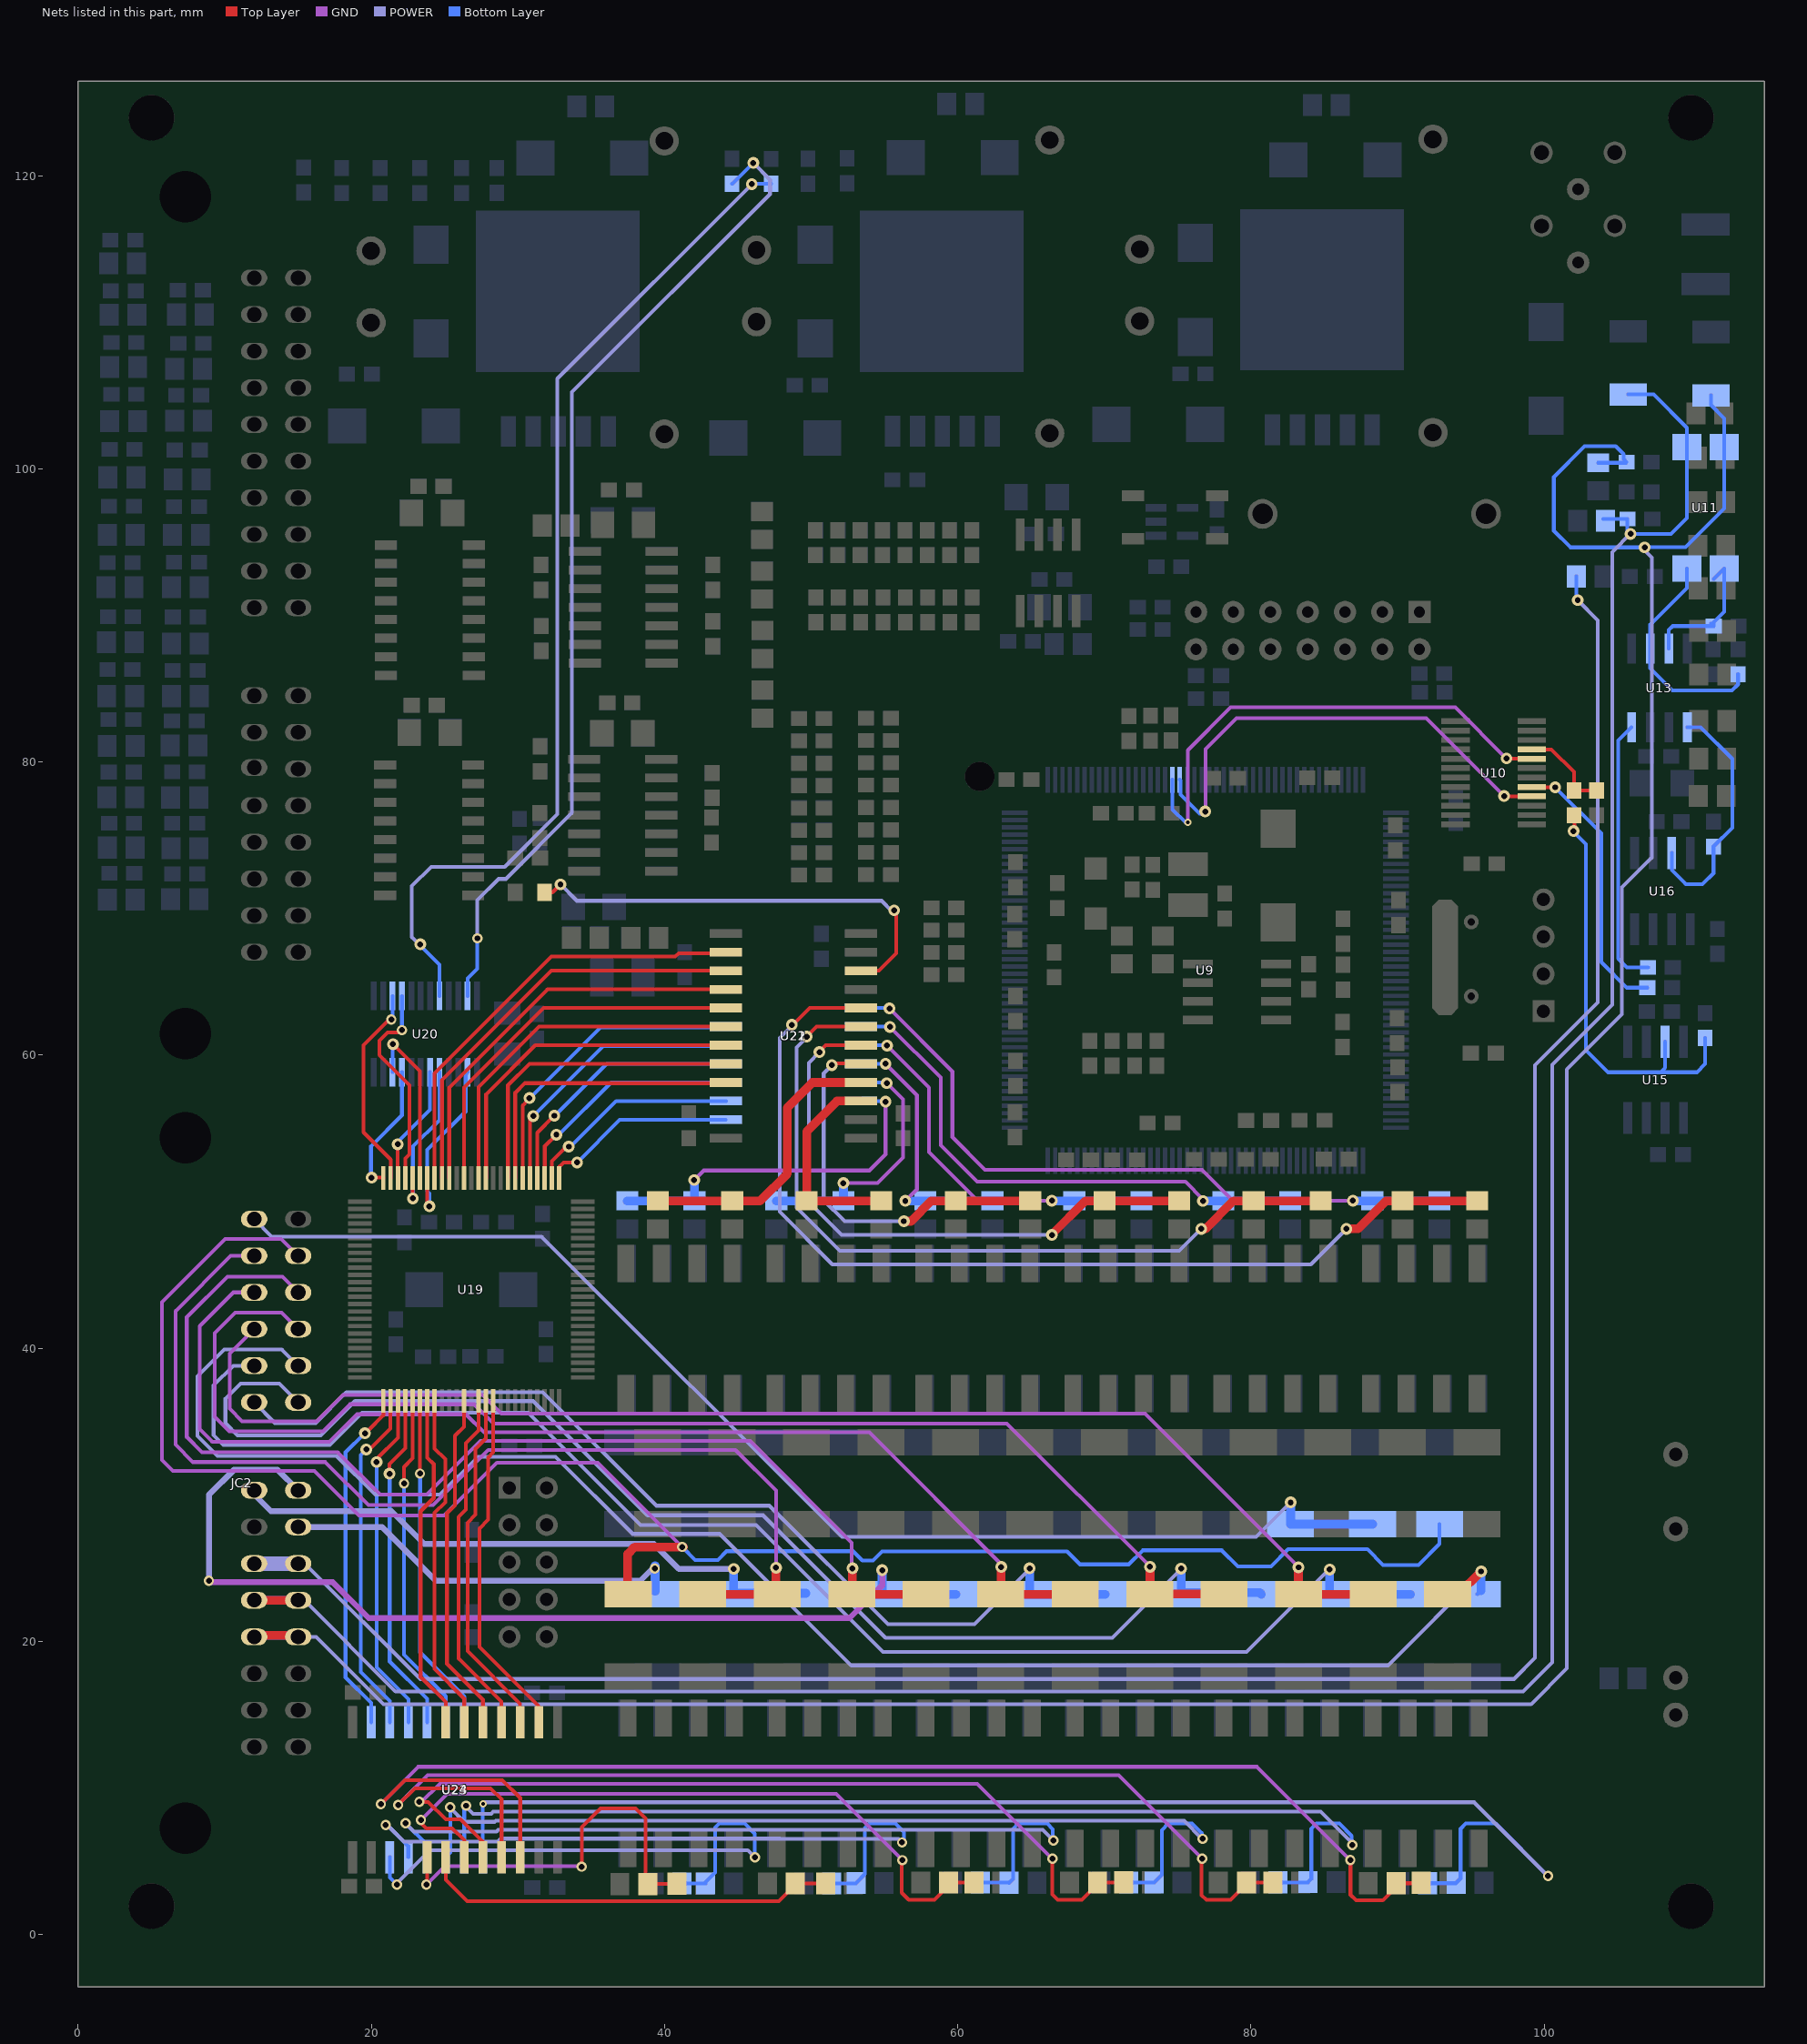
[diagram p0: the nets of this part, all layers, seen from the top]
# Altium PCB MISC86180.PCBDOC (part 5 of 9)
Units mm, origin at the board's own origin, x right, y up, seen from the top; angles counter-clockwise.
Board outline 115 x 130 mm, 4 copper layers (Top Layer, GND, POWER, Bottom Layer); 475 components, 355 nets, 1755 pads, 459 vias.

## Via types
v1: diameter 0.8, hole 0.4, Top Layer to Bottom Layer, 339 vias
v2: diameter 0.7, hole 0.4, Top Layer to Bottom Layer, 83 vias
v3: diameter 0.5, hole 0.254, Top Layer to Bottom Layer, 37 vias

## Nets (pads, with @x,y where several pads share a name; then routed paths per layer and width w, separated by ;. In a path a pad name is that pad's centre, name@x,y a point inside that pad or via, vN(x,y) a via of type N, cw(c..) or ccw(c..) an arc to the next point about the centre after c; other vN are vias at no path point) (continued)
BAT12: F22.1 F23.1 JC2.13 | length 87.7
  POWER w0.254: JC2.13@12.01,48.814 13.204,47.62 31.61,47.62 52.1,27.13 79.851,27.13 79.858,27.137 80.347,27.137 v1(82.7,29.49)
  Bottom Layer w0.254: v1@82.696,29.486 v1(82.7,29.49)
  Bottom Layer w0.6: v1(82.7,29.49) 82.7,28.01 88.28,28.01 F23.1@88.284,28.006
BAT13: F24.1 F25.1 JC2.4 | length 127.3
  Top Layer w0.254: v2@41.2,26.44 v2(41.2,26.45)
  Top Layer w0.6: F25.1@37.484,22.88 37.484,25.954 37.97,26.44 41.2,26.44 v2@41.3,26.44
  GND w0.254: JC2.4@15.01,46.314 13.854,47.47 10.03,47.47 5.71,43.15 5.71,32.39 6.46,31.64 16.11,31.64 19.15,28.6 24.97,28.6 28.57,32.2 35.44,32.2 41.19,26.45 v2(41.2,26.45) ; v2@41.215,26.465 41.22,26.46 v2@41.245,26.435
  Bottom Layer w0.254: v2@41.2,26.44 v2(41.2,26.45) 42.09,25.56 43.63,25.56 44.23,26.16 52.851,26.16 53.488,25.523 54.213,25.523 54.84,26.15 67.45,26.15 68.34,25.26 71.65,25.26 72.61,26.22 78,26.22 79.09,25.13 81.37,25.13 82.53,26.29 87.93,26.29 89,25.22 91.42,25.22 92.856,26.656 F24.1@92.856,28.006
BAT14: F26.1 F27.1 JC2.14 | length 73.7
  Top Layer w0.254: v1@47.6,24.78 v1(47.6,25.03)
  Top Layer w0.6: F26.1@42.604,23.22 F27.1@47.684,23.22 47.6,23.304 v1@47.6,24.78
  GND w0.254: JC2.14@12.01,46.314 10.414,46.314 6.64,42.54 6.64,33.43 7.83,32.24 16.86,32.24 19.8,29.3 24.21,29.3 26.895,31.985 27.98,33.07 44.83,33.07 47.6,30.3 v1(47.6,25.03) ; v1@47.56,25.01 v1@47.56,25.1
BAT15: F28.1 F29.1 JC2.5 | length 77.4
  Top Layer w0.6: v1(52.81,24.99) 52.81,23.266 52.856,23.22 F29.1@57.844,23.22
  GND w0.254: JC2.5@15.01,43.814 13.934,44.89 10.18,44.89 7.41,42.12 7.41,33.95 8.44,32.92 17.71,32.92 20.617,30.013 23.773,30.013 27.44,33.68 45.83,33.68 52.77,26.74 v1@52.77,24.91
BAT16: F30.1 F31.1 JC2.15 | length 78.8
  Top Layer w0.6: v1(62.96,25.08) 62.96,23.256 62.996,23.22 F31.1@68.004,23.22
  GND w0.254: JC2.15@12.01,43.814 10.594,43.814 8.3,41.52 8.3,34.48 9.15,33.63 17.15,33.63 19.02,35.5 26.46,35.5 27.69,34.27 53.97,34.27 62.92,25.32 v1@62.92,25.08
BAT17: F32.1 F33.1 JC2.6 | length 88.8
  Top Layer w0.6: v1(73.11,25.1) 73.11,23.246 78.138,23.246 F33.1@78.164,23.22
  GND w0.254: JC2.6@15.01,41.314 13.884,42.44 10.72,42.44 9.33,41.05 9.33,35.33 10.32,34.34 16.7,34.34 18.54,36.18 27.02,36.18 28.33,34.87 63.35,34.87 v1@73.07,25.15
BAT18: F34.1 F35.1 JC2.16 | length 91.9
  Top Layer w0.6: v1(83.23,25.06) 83.23,23.234 F34.1@83.244,23.22 F35.1@88.324,23.22
  GND w0.254: JC2.16@12.01,41.314 10.34,39.644 10.34,35.88 11.19,35.03 16.28,35.03 18.07,36.82 27.6,36.82 28.87,35.55 72.77,35.55 83.19,25.13 v1@83.19,25.09
BAT19: F36.1 F37.1 JC2.7 | length 115.6
  Top Layer w0.6: F36.1@93.404,23.22 94.13,23.22 v1(95.69,24.78)
  POWER w0.254: JC2.7@15.01,38.814 13.894,39.93 9.97,39.93 8.135,38.095 8.135,34.025 9.5,32.66 17.62,32.66 20.267,30.013 24.693,30.013 27.29,32.61 32.55,32.61 37.82,27.34 43.77,27.34 52.74,18.37 89.34,18.37 v1@95.735,24.765
  Bottom Layer w0.254: F37.1@95.436,23.22 F37.1@95.69,23.474
  Bottom Layer w0.6: F37.1@95.69,23.474 v1(95.69,24.78)
BAT20: F38.1 F39.1 JC2.17 | length 100.5
  POWER w0.254: JC2.17@12.01,38.814 10.584,38.814 9.24,37.47 9.24,34.08 9.92,33.4 17.18,33.4 19.38,35.6 30.71,35.6 38.36,27.95 46.25,27.95 54.91,19.29 79.7,19.29 v1@85.41,25
  Bottom Layer w0.254: F39.1@85.276,23.22 F39.1@85.444,23.22
  Bottom Layer w0.6: v1(85.36,24.91) 85.36,23.304 85.444,23.22 F38.1@90.864,23.22
BAT21: F40.1 F41.1 JC2.8 | length 89.9
  POWER w0.254: JC2.8@15.01,36.314 13.724,37.6 11.08,37.6 10.05,36.57 10.05,34.88 10.87,34.06 16.55,34.06 18.89,36.4 31.05,36.4 38.84,28.61 46.72,28.61 55.07,20.26 70.54,20.26 v1@75.225,24.945
  Bottom Layer w0.6: v1(75.23,24.97) 75.23,23.334 80.59,23.334 F40.1@80.704,23.22
BAT22: F42.1 F43.1 JC2.18 | length 69.4
  POWER w0.254: JC2.18@12.01,36.314 13.414,34.91 16.21,34.91 18.3,37 31.7,37 39.437,29.263 47.137,29.263 55.23,21.17 61.13,21.17 v1@64.96,25
  Bottom Layer w0.254: F43.1@64.9,23.276 F43.1@64.956,23.22
  Bottom Layer w0.6: F43.1@64.9,23.276 v1(64.9,24.99) ; F43.1@64.956,23.22 F42.1@70.036,23.22
BAT23: F44.1 F45.1 JC2.9 | length 69.2
  GND w0.4: v2(8.92,24.14) 9.01,24.05 17.36,24.05 19.82,21.59 52.61,21.59 54.84,23.82 v1(54.84,24.87)
  POWER w0.254: v1@54.74,24.82 v1@54.94,24.82
  POWER w0.4: v2(8.92,24.14) 8.92,30 10.65,31.73 13.594,31.73 JC2.9@15.01,30.314
  Bottom Layer w0.254: F45.1@54.796,23.22 F45.1@54.884,23.22
  Bottom Layer w0.6: v1(54.84,24.87) 54.84,23.264 54.884,23.22 F44.1@59.876,23.22
BAT24: F46.1 F47.1 JC2.19 | length 41.9
  POWER w0.4: JC2.19@12.01,30.314 12.01,30.03 13.154,28.885 21.375,28.885 23.605,26.655 39.265,26.655 40.97,24.95 v1(44.71,24.95)
  Bottom Layer w0.254: v1@44.636,24.876 v1(44.71,24.95) ; F46.1@49.642,23.22 F46.1@49.716,23.22
  Bottom Layer w0.6: v1(44.71,24.95) 44.71,23.294 F46.1@49.642,23.294
BAT25: F48.1 JC2.10 | length 27.9
  POWER w0.4: JC2.10@15.01,27.814 20.726,27.814 24.4,24.14 38.34,24.14 39.18,24.98 v2(39.33,24.98)
  Bottom Layer w0.254: v2@39.342,25.163 v2@39.349,25.17
  Bottom Layer w0.6: F48.1@39.35,23.426 v2@39.35,25.17
CAN1H: C60.2 DZ1.1 JC2.23 JC2.31 R17.2 U11.4 | length 209.4
  Top Layer w0.6: JC2.31@12.01,20.414 JC2.23@14.91,20.414
  POWER w0.254: JC2.23@15.01,20.314 16.236,20.314 20.83,15.72 99.1,15.72 101.54,18.16 101.54,52.89 ; 101.54,54.63 101.54,52.89 ; 105.29,69.915 105.29,71.39 105.3,71.4 105.3,71.44 107.34,73.48 107.34,93.942 106.85,94.432 v1(106.85,94.64) ; 105.3,69.861 105.3,62.78 101.54,59.02 101.54,52.89
  Bottom Layer w0.254: R17.2@103.672,100.409 105.557,100.409 C60.2@105.61,100.462 105.41,100.662 105.41,101 104.87,101.54 102.75,101.54 100.65,99.44 100.65,95.76 101.77,94.64 v1(106.85,94.64) ; v1@106.85,94.65 109.62,94.65 112.263,97.293 U11.4@112.263,101.485 112.263,103.447 111.36,104.35 DZ1.1@111.36,105.012
  Bottom Layer w0.6: JC2.31@12.01,20.414 JC2.23@14.91,20.414
CAN1HIN: C58.2 U11.1 U13.7 | length 9.9
  Bottom Layer w0.254: U13.7@108.49,87.727 108.49,89.01 108.752,89.272 C58.2@111.55,89.272 ; C58.2@111.382,89.44 C58.2@111.55,89.272 ; U11.1@111.55,92.472 U11.1@112.263,93.185 112.263,90.243 111.55,89.53 C58.2@111.55,89.272
CAN1L: C61.2 DZ2.1 JC2.22 JC2.30 R18.1 U11.3 | length 192.4
  Top Layer w0.6: JC2.30@12.01,22.814 JC2.22@15.01,22.814
  POWER w0.254: JC2.22@15.01,22.814 15.426,22.814 21.65,16.59 98.55,16.59 100.53,18.57 100.53,59.34 104.63,63.44 104.63,94.32 v1@105.95,95.64
  Bottom Layer w0.254: R18.1@104.019,96.582 C61.2@105.67,96.582 105.67,95.77 105.89,95.55 108.64,95.55 109.723,96.633 U11.3@109.723,101.485 109.723,102.799 107.45,105.072 DZ2.1@105.72,105.072
  Bottom Layer w0.6: JC2.30@12.01,22.814 JC2.22@15.01,22.814
  other v1: 105.89,95.56
CAN1LIN: C59.2 U11.2 U13.6 | length 15.3
  Bottom Layer w0.254: U11.2@109.723,93.185 109.723,91.863 107.23,89.37 107.23,87.737 U13.6@107.22,87.727 107.22,86.39 108.62,84.99 108.73,84.88 112.8,84.88 113.218,85.298 C59.2@113.218,85.99
CAN1RX: R22.2 U13.4 | length 18.5
  Bottom Layer w0.254: U13.4@105.95,82.377 105.03,81.457 105.03,66.59 105.63,65.99 107.062,65.99 R22.2@107.07,65.982
CAN1S: JC2.21 JC2.29 R19.2 | length 167.4
  POWER w0.254: JC2.21@15.01,25.314 15.476,25.314 23.35,17.44 97.93,17.44 99.37,18.88 99.37,59.32 103.65,63.6 103.65,89.67 v1(102.28,91.04)
  POWER w1: JC2.29@12.01,25.314 JC2.21@15.01,25.314
  Bottom Layer w0.254: R19.2@102.175,92.658 102.175,91.145 v1(102.28,91.04)
CAN1TX: R23.1 U13.1 U16.7 | length 17
  Bottom Layer w0.254: U16.7@108.693,73.791 108.693,72.617 109.65,71.66 110.79,71.66 111.542,72.412 R23.1@111.542,74.23 112.83,75.518 112.83,80.21 110.663,82.377 U13.1@109.76,82.377
CANAR: R13.1 R14.2 U10.9 | length 6.3
  Top Layer w0.254: U10.9@99.146,80.858 100.482,80.858 102.022,79.318 R13.1@102.022,78.06 R14.2@103.568,78.06
CANARR: R13.2 R21.1 U15.7 | length 29.6
  Top Layer w0.254: v1@101.82,75.11 v1@101.852,75.142 ; v1@102.07,75.16 R13.2@102.07,76.378
  Bottom Layer w0.254: v1@101.82,75.11 102.11,75.11 102.83,74.39 102.83,60.35 104.35,58.83 107.92,58.83 ; U15.7@108.231,60.913 108.231,59.141 107.92,58.83 ; R21.1@110.972,61.17 110.972,59.402 110.4,58.83 107.92,58.83
  other v1: 101.99,75.29
CANARX: U9.62 U10.8 | length 34.5
  Top Layer w0.254: v1(97.42,80.24) 97.442,80.218 U10.8@99.146,80.218
  GND w0.254: v3(75.68,75.87) 75.68,80.8 78.6,83.72 93.94,83.72 v1(97.42,80.24)
  Bottom Layer w0.254: U9.62@74.639,78.793 74.639,76.761 75.53,75.87 v3(75.68,75.87)
CANAT: R24.2 U10.5 | length 20.6
  Top Layer w0.254: U10.5@99.146,78.298 99.175,78.27 v1(100.74,78.27)
  Bottom Layer w0.254: v1(100.74,78.27) 103.88,75.13 103.88,66.34 105.618,64.602 ; 104.27,65.95 105.618,64.602 ; R24.2@107.02,64.602 105.618,64.602
CANATX: U9.63 U10.4 | length 33.4
  Top Layer w0.254: v1(97.26,77.67) 97.272,77.658 U10.4@99.146,77.658
  GND w0.254: v1(76.87,76.62) 77.026,76.464 76.9,76.59 76.9,80.88 79,82.98 91.95,82.98 v1(97.26,77.67)
  Bottom Layer w0.254: U9.63@75.139,78.793 75.184,78.748 75.184,77.778 76.499,76.463 76.838,76.463 76.87,76.496 v1(76.87,76.62)
CI1: U19.69 U20.2 | length 12.6
  Top Layer w0.254: U19.69@23.816,51.614 23.816,49.824 v1@24.126,49.514
  Bottom Layer w0.254: v1(23.96,49.69) 23.964,49.694 23.964,50.566 23.82,50.71 23.82,53.54 26.432,56.152 26.432,58.707 U20.2@26.568,58.842
CI2: U19.70 U20.10 | length 11.8
  Top Layer w0.254: v1(21.47,60.75) 23.316,58.904 U19.70@23.316,51.614
  Bottom Layer w0.254: U20.10@21.47,58.864 U20.10@21.448,58.842 21.448,60.728 v1(21.47,60.75)
CI3: U19.71 U20.5 | length 10.9
  Top Layer w0.254: v1@22.816,50.276 U19.71@22.816,51.614
  Bottom Layer w0.254: v1@22.66,50.06 v1(22.83,50.23) 22.83,53.75 24.648,55.568 U20.5@24.648,58.842
CI4: U19.72 U20.16 | length 14.5
  Top Layer w0.254: v2@22.08,61.7 21.93,61.55 21.11,61.55 20.54,60.98 20.54,60.01 22.6,57.95 22.6,53.23 22.316,52.946 U19.72@22.316,51.614
  Bottom Layer w0.254: v2@22.08,61.7 v2(22.088,61.708) U20.16@22.088,64.042
CI5: U19.73 U20.6 | length 8
  Top Layer w0.254: v1(21.8,53.92) 21.8,51.63 U19.73@21.816,51.614
  Bottom Layer w0.254: v1@21.8,54.07 24.008,56.278 U20.6@24.008,58.842
CI6: U19.74 U20.15 | length 14.1
  Top Layer w0.254: U19.74@21.316,51.614 21.316,52.874 19.453,54.737 19.453,60.676 21.206,62.43 v2(21.36,62.43)
  Bottom Layer w0.254: v2(21.36,62.43) 21.448,62.517 U20.15@21.448,64.042
CI7: U19.75 U20.9 | length 8.9
  Top Layer w0.254: v1(20.02,51.64) 20.79,51.64 U19.75@20.816,51.614
  Bottom Layer w0.254: v1@19.98,51.64 19.98,53.8 22.088,55.908 U20.9@22.088,58.842
CI9: R96.1 U20.23 | length 68.2
  POWER w0.254: v2(27.23,67.97) 27.23,70.58 28.67,72.02 29.18,72.02 33.68,76.52 33.68,105.23 47.19,118.74 47.19,119.73 v1(46.05,120.87)
  Bottom Layer w0.254: U20.23@26.568,64.042 26.568,65.228 27.23,65.89 v2(27.23,67.97) ; R96.1@44.61,119.452 44.632,119.452 v1(46.05,120.87)
CI10: R97.1 U20.20 | length 70
  POWER w0.254: v1(23.34,67.56) 23.25,67.56 22.76,68.05 22.76,71.53 24.08,72.85 29.1,72.85 32.68,76.43 32.68,106.15 v1(45.95,119.42)
  Bottom Layer w0.254: v1(23.34,67.56) 23.34,67.47 24.648,66.162 U20.20@24.648,64.042 ; v1@45.972,119.442 R97.1@47.256,119.442
CO1: U19.66 U22.16 | length 27.8
  Top Layer w0.254: U19.66@25.316,51.614 25.316,57.786 32.019,64.489 U22.16@44.192,64.489
CO2: U19.64 U22.17 | length 26.3
  Top Layer w0.254: U19.64@26.316,51.614 26.316,57.786 31.749,63.219 U22.17@44.192,63.219
CO3: U19.62 U22.18 | length 24.8
  Top Layer w0.254: U19.62@27.316,51.614 27.316,57.826 31.439,61.949 U22.18@44.192,61.949
CO4: U19.61 U22.19 | length 23.5
  Top Layer w0.254: U19.61@27.83,51.628 27.83,57.33 31.179,60.679 U22.19@44.192,60.679
CO5: U19.57 U22.21 | length 20.4
  Top Layer w0.254: U19.57@29.816,51.614 29.816,57.436 30.47,58.09 U22.21@44.143,58.09
CO6: U19.58 U22.20 | length 21.8
  Top Layer w0.254: U19.58@29.316,51.614 29.316,57.936 30.789,59.409 U22.20@44.192,59.409
CO7: U19.51 U21.14 | length 13.4
  Top Layer w0.254: U19.51@32.816,51.614 32.816,52.376 33.12,52.68 v1(34.03,52.68)
  Bottom Layer w0.254: v1@34.035,52.675 36.94,55.58 U21.14@44.173,55.58
CO8: U19.52 U21.15 | length 14.1
  Top Layer w0.254: U19.52@32.316,51.614 32.316,52.766 v1@33.15,53.6
  Bottom Layer w0.254: v1@33.71,53.88 36.699,56.869 U21.15@44.192,56.869
  other v1: 33.47,53.76
CO9: U19.53 U21.16 | length 16.2
  Top Layer w0.254: U19.53@31.83,51.718 31.83,53.78 v1(32.62,54.57)
  Bottom Layer w0.254: v1(32.62,54.57) 32.79,54.57 36.359,58.139 U21.16@44.192,58.139
CO10: U19.54 U21.17 | length 17.9
  Top Layer w0.254: U19.54@31.316,51.614 31.316,54.706 v1(32.48,55.87)
  Bottom Layer w0.254: v1@32.495,55.855 36.049,59.409 U21.17@44.192,59.409
CO11: U19.55 U21.18 | length 19.4
  Top Layer w0.254: U19.55@30.816,51.614 30.816,55.606 v1(31.05,55.84)
  Bottom Layer w0.254: v1(31.05,55.84) 35.83,60.62 U21.18@44.133,60.62
CO12: U19.56 U21.19 | length 21
  Top Layer w0.254: U19.56@30.316,51.614 30.316,56.566 v1@30.64,56.89
  Bottom Layer w0.254: v1@30.64,56.89 35.63,61.88 U21.19@44.123,61.88
  other v1: 30.78,57.07
CO13: U19.7 U23.19 | length 23.2
  Top Layer w0.254: U19.7@23.816,36.414 23.816,32.544 24.26,32.1 24.26,29.79 23.36,28.89 23.36,17.58 25.069,15.871 U23.19@25.069,14.492
CO14: U19.8 U23.18 | length 23.4
  Top Layer w0.254: U19.8@24.316,36.414 24.316,33.164 25.045,32.435 25.045,29.505 24.31,28.77 24.31,18.13 26.339,16.101 U23.18@26.339,14.492
CO15: U19.12 U23.17 | length 22.8
  Top Layer w0.254: U19.12@26.316,36.414 26.316,34.656 25.7,34.04 25.7,29.29 25.16,28.75 25.16,18.48 27.609,16.031 U23.17@27.609,15.101
CO16: U19.14 U23.16 | length 23.7
  Top Layer w0.254: U19.14@27.316,36.414 27.316,34.41 26.44,33.534 26.44,28.99 25.94,28.49 25.94,18.84 28.879,15.901 U23.16@28.879,14.492
CO17: U19.15 U23.15 | length 23.9
  Top Layer w0.254: U19.15@27.816,36.414 27.816,33.856 27.1,33.14 27.1,28.65 26.56,28.11 26.56,19.34 30.149,15.751 U23.15@30.149,14.492
CO18: U19.16 U23.14 | length 24
  Top Layer w0.254: U19.16@28.316,36.414 28.316,32.896 27.97,32.55 27.97,28.31 27.37,27.71 27.37,19.63 31.419,15.581 U23.14@31.419,14.492
CO19: U19.6 U24.19 | length 23.2
  Top Layer w0.254: U19.6@23.316,36.414 v2(23.316,31.454) v2@23.45,31.32
  Bottom Layer w0.254: v2@23.33,31.32 23.33,19.24 26.339,16.231 U24.19@26.339,14.492
CO20: U19.5 U24.18 | length 23.3
  Top Layer w0.254: v2@22.22,30.79 22.22,31.9 22.816,32.496 U19.5@22.816,36.414
  Bottom Layer w0.254: v2@22.22,30.79 22.22,19.11 25.069,16.261 U24.18@25.069,14.492
  other v2: 22.23,30.79
CO21: U19.4 U24.17 | length 23.4
  Top Layer w0.254: v1@21.24,31.2 21.24,32.11 22.316,33.186 U19.4@22.316,36.414
  Bottom Layer w0.254: v1@21.25,31.2 21.25,18.63 23.799,16.081 U24.17@23.799,14.492
  other v1: 21.24,31.44
CO22: U19.3 U24.16 | length 23.4
  Top Layer w0.254: v1@20.38,32.01 20.38,32.46 21.816,33.896 U19.3@21.816,36.414
  Bottom Layer w0.254: v1@20.36,32.01 20.36,18.22 22.529,16.051 U24.16@22.529,14.492
  other v1: 20.36,32.24
CO23: U19.2 U24.15 | length 23.9
  Top Layer w0.254: v1@19.49,32.93 19.72,32.93 21.3,34.51 U19.2@21.3,36.398
  Bottom Layer w0.254: v1(19.66,33.1) 19.279,32.719 19.279,17.92 21.259,15.94 U24.15@21.259,14.492
CO24: U19.1 U24.14 | length 23.4
  Top Layer w0.254: v1@19.79,34.41 20.82,35.44 U19.1@20.82,36.37
  Bottom Layer w0.254: v1(19.57,34.21) 19.57,34.19 19.53,34.19 18.24,32.9 18.24,17.55 19.989,15.801 U24.14@19.989,14.492
CO25: U19.67 U22.15 | length 29.1
  Top Layer w0.254: U19.67@24.816,51.614 24.816,58.296 32.279,65.759 U22.15@44.192,65.759
CO26: U19.68 U22.14 | length 30.4
  Top Layer w0.254: U19.68@24.316,51.614 24.316,58.756 32.28,66.72 40.73,66.72 40.967,66.957 44.12,66.957 U22.14@44.192,67.029
CT1: R33.2 R34.2 U22.8 | length 69.2
  Top Layer w0.254: v1(48.68,62.07) 48.75,62.07 49.899,63.219 U22.8@53.392,63.219 ; v1(86.5,48.15) v1@86.52,48.13 ; 87.28,48.13 87.3,48.13
  Top Layer w0.6: v1(86.5,48.15) 87.28,48.15 ; 87.3,48.15 89.203,50.053 R34.2@90.334,50.053 R33.2@95.414,50.053
  POWER w0.254: v1(48.68,62.07) 48.68,62 47.85,61.17 47.85,49.32 51.44,45.73 84.08,45.73 v1(86.5,48.15)
CT2: R35.2 R36.2 U22.7 | length 54.5
  Top Layer w0.254: v1(49.69,61.26) 50.379,61.949 U22.7@53.392,61.949 ; v1(76.6,48.15) v1@76.71,48.15 ; 78.613,50.053 78.8,50.053
  Top Layer w0.6: v1@76.71,48.15 76.897,48.15 78.8,50.053 R36.2@80.174,50.053 R35.2@84.746,50.053
  POWER w0.254: v1(49.69,61.26) 49.69,61.22 49,60.53 49,49.61 51.96,46.65 75.1,46.65 v1(76.6,48.15)
CT3: R37.2 R38.2 U22.6 | length 40.8
  Top Layer w0.254: v1(50.56,60.21) 50.56,60.25 51,60.69 53.381,60.69 U22.6@53.392,60.679
  Top Layer w0.6: v1@66.395,47.755 68.693,50.053 R38.2@70.014,50.053 R37.2@75.094,50.053
  POWER w0.254: v1(50.56,60.21) 49.83,59.48 49.83,49.98 52.08,47.73 v1(66.42,47.73)
CT4: R41.2 R42.2 U22.5 | length 26.8
  Top Layer w0.254: v1(51.41,59.32) 51.41,59.34 51.5,59.43 53.371,59.43 U22.5@53.392,59.409 ; v1(56.32,48.67) v1@56.32,48.7
  Top Layer w0.6: v1(56.32,48.67) 56.81,48.67 58.193,50.053 R42.2@59.854,50.053 R41.2@64.934,50.053
  POWER w0.254: v1(51.41,59.32) 50.85,58.76 50.85,50.11 52.29,48.67 v1(56.32,48.67)
CT5: R43.2 R44.2 U22.3 | length 14.4
  Top Layer w0.6: U22.3@53.392,56.869 51.769,56.869 49.694,54.794 R44.2@49.694,50.053 R43.2@54.774,50.053
CT6: R45.2 R46.2 U22.4 | length 20.1
  Top Layer w0.254: 46.513,50.053 46.723,50.053
  Top Layer w0.6: R46.2@39.534,50.053 R45.2@44.614,50.053 46.513,50.053 48.37,51.91 48.37,56.42 50.089,58.139 U22.4@53.392,58.139
CT7: R47.2 R48.2 U21.10 | length 25
  GND w0.254: v1(42.02,51.48) 42.67,52.13 53.96,52.13 55.07,53.24 v1(55.07,56.82)
  Bottom Layer w0.254: U21.10@53.392,56.869 v1@55.021,56.869
  Bottom Layer w0.6: R47.2@37.466,50.053 R48.2@42.038,50.053 v1@42.038,51.462
CT8: R49.2 R50.2 U21.9 | length 17.9
  GND w0.254: v1(52.19,51.27) 54.52,51.27 56.26,53.01 56.26,56.98 v1(55.15,58.09)
  Bottom Layer w0.254: U21.9@53.392,58.139 55.101,58.139 v1(55.15,58.09)
  Bottom Layer w0.6: R49.2@47.626,50.053 R50.2@52.198,50.053 v1@52.198,51.262
CT9: R51.2 R52.2 U21.8 | length 18.2
  GND w0.254: v1(55.07,59.41) 55.07,59.4 57.21,57.26 57.21,50.85 v1(56.42,50.06)
  Bottom Layer w0.254: U21.8@53.392,59.409 v1(55.07,59.41) ; v1(56.42,50.06) v1@56.427,50.053
  Bottom Layer w0.6: v1@56.427,50.053 R51.2@57.786,50.053 R52.2@62.358,50.053
CT10: R53.2 R54.2 U21.7 | length 26.1
  GND w0.254: v1(55.17,60.65) 58.04,57.78 58.04,53.38 61.35,50.07 v1(66.42,50.07)
  Bottom Layer w0.254: U21.7@53.392,60.679 55.141,60.679 v1(55.17,60.65) ; v1(66.42,50.07) v1@66.437,50.07
  Bottom Layer w0.6: v1@66.437,50.053 R53.2@67.946,50.053 R54.2@72.518,50.053
CT11: R55.2 R56.2 U21.6 | length 37
  GND w0.254: v1(55.37,61.93) 58.83,58.47 58.83,53.84 61.31,51.36 75.52,51.36 76.72,50.16 v1(76.72,50.05)
  Bottom Layer w0.254: U21.6@53.392,61.949 55.351,61.949 v1(55.37,61.93)
  Bottom Layer w0.6: v1@76.723,50.053 R55.2@78.106,50.053 R56.2@82.678,50.053
CT12: R57.2 R58.2 U21.5 | length 47.5
  GND w0.254: v1(55.34,63.18) 59.63,58.89 59.63,54.4 61.85,52.18 76.66,52.18 78.77,50.07 v1(86.94,50.07)
  Bottom Layer w0.254: U21.5@53.392,63.219 55.301,63.219 v1(55.34,63.18)
  Bottom Layer w0.6: v1@86.957,50.053 R57.2@88.266,50.053 R58.2@92.838,50.053
CT13: R59.2 R60.2 U23.5 | length 27.4
  Top Layer w0.254: v2(23.75,3.41) 23.805,3.465 U23.5@23.805,5.28 ; v2(34.35,4.64) 34.35,7.34 35.62,8.61 38.02,8.61 38.71,7.92 38.71,4.06 38.849,3.921 R59.2@38.849,3.452 40.814,3.452 R60.2@40.841,3.478
  GND w0.254: v2(23.75,3.41) 25.01,4.67 34.32,4.67 v2(34.35,4.64)
CT14: R61.2 R62.2 U23.6 | length 28.6
  Top Layer w0.254: U23.6@25.075,5.28 25.075,3.745 26.545,2.275 47.796,2.275 48.919,3.398 R61.2@48.919,3.502 50.987,3.502 R62.2@50.991,3.498
CT15: R63.2 R64.2 U23.7 | length 48.2
  Top Layer w0.254: v2(23.38,7.82) 23.38,7.63 23.75,7.26 25.52,7.26 26.345,6.435 U23.7@26.345,5.28 ; v2(56.22,5.08) 56.18,5.04 56.18,2.857 56.652,2.385 58.415,2.385 59.379,3.349 R63.2@59.379,3.562 61.087,3.562 R64.2@61.101,3.548
  GND w0.254: v2(23.38,7.82) 25.167,9.607 51.693,9.607 v2(56.22,5.08)
CT16: R65.2 R66.2 U23.8 | length 60.4
  Top Layer w0.254: v2(23.28,9.06) 23.88,9.06 25.07,7.87 26.07,7.87 27.615,6.325 U23.8@27.615,5.28 ; v2(66.45,5.18) 66.44,5.17 66.44,2.747 66.802,2.385 68.456,2.385 69.529,3.458 R65.2@69.529,3.562 R66.2@71.304,3.562
  Top Layer w0.6: R66.2@71.304,3.562 R66.2@71.311,3.568
  GND w0.254: v2(23.28,9.06) 23.33,9.01 23.38,9.01 24.67,10.3 61.33,10.3 v2(66.45,5.18)
CT17: R67.2 R68.2 U23.9 | length 78.4
  Top Layer w0.254: v2(21.83,8.85) 22.96,9.98 28.13,9.98 28.885,9.225 U23.9@28.885,5.28 ; v2(76.67,5.18) 76.63,5.22 76.63,2.697 76.952,2.375 78.606,2.375 79.679,3.448 R67.2@79.679,3.552 ; R67.2@79.579,3.652 R67.2@79.679,3.552 ; R68.2@81.481,3.269 R68.2@81.481,3.558 81.474,3.552 R67.2@79.679,3.552
  GND w0.254: v2(21.83,8.85) 23.85,10.87 70.98,10.87 v2(76.67,5.18)
CT18: R69.2 R70.2 U23.10 | length 93
  Top Layer w0.254: v2(20.65,8.9) 22.29,10.54 28.93,10.54 30.155,9.315 U23.10@30.155,5.28 ; v2(86.77,5.09) 86.78,5.08 86.78,2.717 87.162,2.335 88.985,2.335 89.889,3.239 R69.2@89.889,3.512 ; R69.2@89.889,3.961 R69.2@89.889,3.512 ; R70.2@91.611,3.538 91.584,3.512 R69.2@89.889,3.512
  GND w0.254: v2(20.65,8.9) 23.2,11.45 80.41,11.45 v2(86.77,5.09)
CT19: R71.2 R72.2 U24.5 | length 91.8
  POWER w0.254: v3(27.63,8.93) 27.73,9.03 95.22,9.03 v2@100.245,4.005
  Bottom Layer w0.254: U24.5@27.609,5.292 27.6,5.301 27.6,8.9 v3(27.63,8.93) ; R72.2@92.039,3.508 93.957,3.508 R71.2@93.991,3.542 94.29,3.841 94.29,7.23 94.641,7.581 96.679,7.581 v2(100.26,4)
CT20: R73.2 R74.2 U24.6 | length 75.1
  POWER w0.254: v2(26.46,8.8) 26.46,8.74 26.947,8.253 28.182,8.253 28.319,8.39 84.76,8.39 86.83,6.32 v2@86.83,6.05
  Bottom Layer w0.254: U24.6@26.339,5.292 26.339,8.679 v2(26.46,8.8) ; R74.2@81.839,3.568 83.867,3.568 R73.2@83.891,3.592 84.11,3.811 84.11,7.22 84.471,7.581 86.024,7.581 86.87,6.735 86.87,6.13 86.88,6.12 v2(86.9,6.12)
CT21: R75.2 R76.2 U24.7 | length 65.1
  POWER w0.254: v2(25.38,8.69) 25.38,8.65 26.331,7.699 28.411,7.699 28.482,7.77 75.43,7.77 76.66,6.54 v2@76.81,6.54
  Bottom Layer w0.254: U24.7@25.069,5.292 25.38,5.603 v2(25.38,8.69) ; R76.2@71.659,3.548 73.387,3.548 R75.2@73.391,3.552 73.92,4.081 73.92,7.133 74.368,7.581 75.979,7.581 76.64,6.92 76.64,6.56 76.66,6.54 v2(76.7,6.54)
CT22: R77.2 R78.2 U24.8 | length 57.3
  POWER w0.254: v2@22.35,7.59 22.897,7.043 28.539,7.043 28.646,7.15 65.79,7.15 v2@66.56,6.38
  Bottom Layer w0.254: v2(22.33,7.6) 22.332,7.6 23.799,6.133 U24.8@23.799,5.292 ; R78.2@61.539,3.558 63.484,3.558 R77.2@63.501,3.542 63.77,3.811 63.77,7.23 64.121,7.581 66.089,7.581 66.48,7.19 66.48,6.47 v2(66.52,6.43)
CT23: R79.2 R80.2 U24.9 | length 48.2
  POWER w0.254: v2(20.98,7.48) 21.09,7.48 22.229,6.341 28.62,6.341 28.829,6.55 47.86,6.55 ; 47.86,6.54 55.95,6.54 v2(56.2,6.29)
  Bottom Layer w0.254: v2(20.98,7.48) 21.075,7.48 22.52,6.035 22.52,5.301 U24.9@22.529,5.292 ; R80.2@51.389,3.488 R79.2@53.027,3.488 ; R79.2@53.071,3.532 53.67,4.131 53.67,7.27 53.981,7.581 55.739,7.581 56.33,6.99 56.33,6.36 56.26,6.29 v2(56.2,6.29)
CT24: R81.2 R82.2 U24.10 | length 38.2
  POWER w0.254: v2(21.74,3.41) 21.74,3.5 24,5.76 45.67,5.76 v2@46.175,5.255
  Bottom Layer w0.254: U24.10@21.27,5.303 U24.10@21.259,5.292 21.259,3.891 v2(21.74,3.41) ; R82.2@41.189,3.498 R81.2@42.794,3.498 ; R81.2@42.801,3.492 42.801,3.591 43.46,4.25 43.46,7.32 43.721,7.581 45.469,7.581 46.16,6.89 46.16,5.28 v2(46.17,5.27)
CT25: L1.1 U22.10 | length 30.8
  Top Layer w0.254: L1.1@31.815,71.108 32.358,71.108 v1(32.9,71.65) ; U22.10@53.392,65.759 54.619,65.759 55.8,66.94 55.8,69.74 v1(55.66,69.88)
  POWER w0.254: v1(32.9,71.65) 34.02,70.53 54.8,70.53 55.52,69.81 55.59,69.81 v1(55.66,69.88)